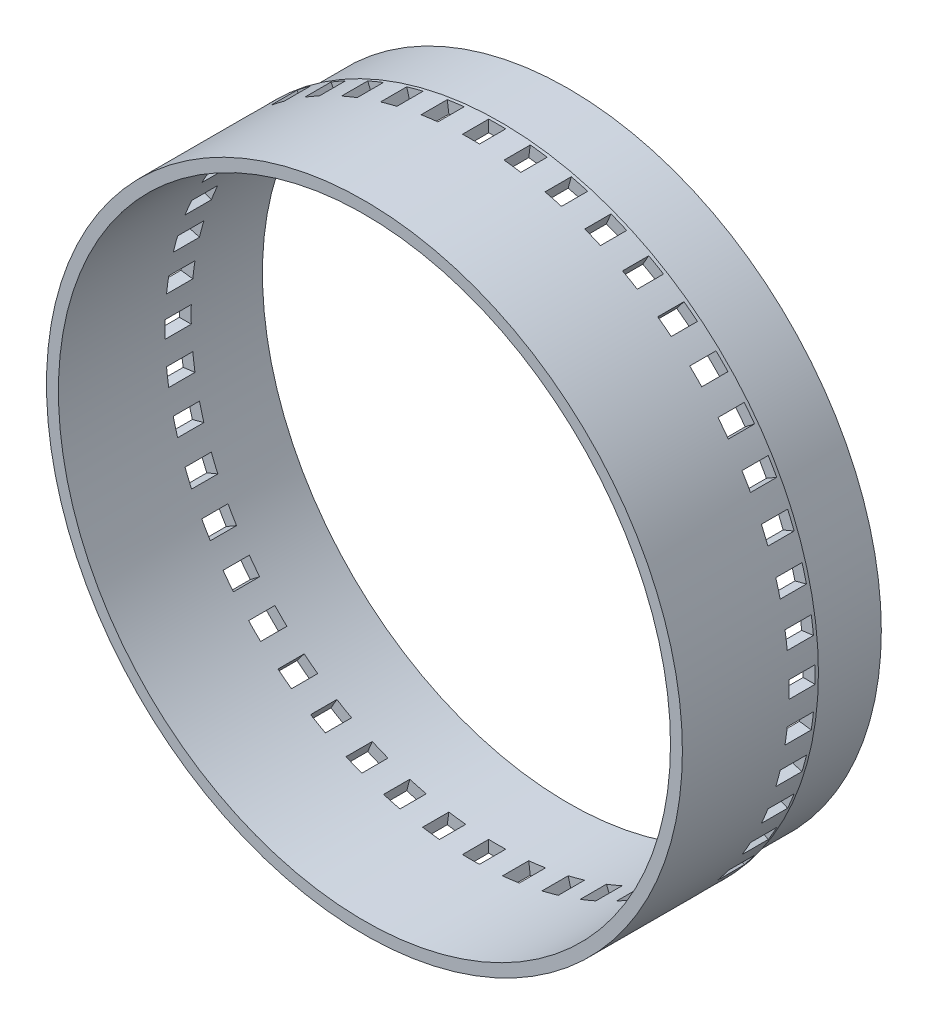
SolidWorks part; units mm, degrees
ref_plane "Front Plane" through (0, 0, 0) normal (0, 0, 1) x (1, 0, 0)
ref_plane "Top Plane" through (0, 0, 0) normal (0, 1, 0) x (1, 0, 0)
ref_plane "Right Plane" through (0, 0, 0) normal (1, 0, 0) x (0, 0, -1)
sketch "Sketch1" plane through (0, 0, 0) normal (0, 0, 1) x (1, 0, 0)
  circle A0 centre (0, 0) radius 9.2
  dimension "D1" = 18.4
extrude "Boss-Extrude1" add sketch "Sketch1" along normal blind 2
sketch "Sketch2" plane through (0, 0, 2) normal (0, 0, 1) x (1, 0, 0)
  circle A0 centre (0, 0) radius 9.35
  dimension "D1" = 18.7
extrude "Boss-Extrude2" add sketch "Sketch2" along normal blind 4
sketch "Sketch3" plane through (0, 0, 6) normal (0, 0, 1) x (1, 0, 0)
  circle A0 centre (0, 0) radius 9
  dimension "D1" = 18
extrude "Cut-Extrude1" cut sketch "Sketch3" against normal blind 13
sketch "Sketch4" plane through (0, 0, 0) normal (0, 1, 0) x (1, 0, 0)
  line L1 (-8.988, -2.0956) -> (-9.5328, -2.0956)
  line L2 (-8.988, -2.0956) -> (-8.988, -2.8672)
  line L3 (-8.988, -2.8672) -> (-9.5328, -2.8672)
  line L4 (-9.5328, -2.0956) -> (-9.5328, -2.8672)
extrude "Cut-Extrude2" cut sketch "Sketch4" against normal mid plane 0.5
pattern_circular "CirPattern1" count 48 over 360 about axis through (0, 0, 0) along (0, 0, 1) of "Cut-Extrude2"
